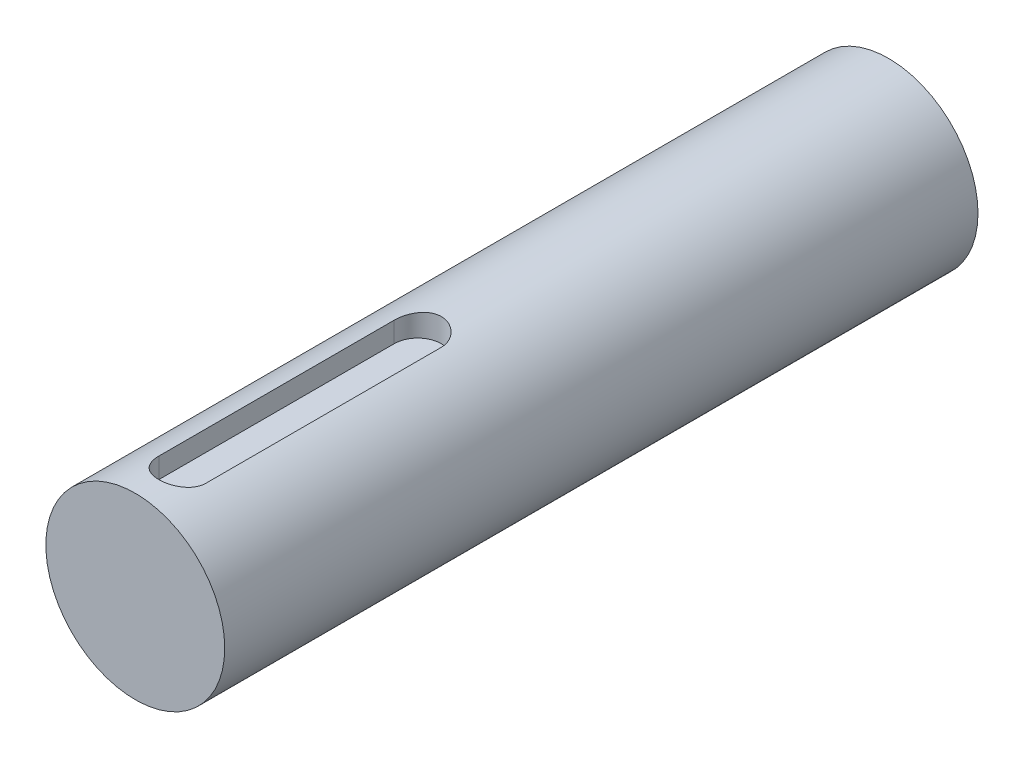
SolidWorks part; units mm, degrees
ref_plane "Front Plane" through (0, 0, 0) normal (0, 0, 1) x (1, 0, 0)
ref_plane "Top Plane" through (0, 0, 0) normal (0, 1, 0) x (1, 0, 0)
ref_plane "Right Plane" through (0, 0, 0) normal (1, 0, 0) x (0, 0, -1)
sketch "Sketch 1" plane through (0, 0, 0) normal (0, 0, 1) x (1, 0, 0)
  circle A0 centre (0, 0) radius 19
  dimension "D1" = 38
extrude "Boss-Extrude 1" add sketch "Sketch 1" along normal blind 160
ref_plane "Plane 1" through (0, 14, 0) normal (0, 1, 0) x (1, 0, 0)
sketch "Sketch 3" plane through (0, 14, 0) normal (0, 1, 0) x (1, 0, 0)
  line L0 (0, -33.0868) -> (0, -201.8775) construction
  line L1 (0, -150) -> (0, -100) construction
  line L2 (-5, -150) -> (-5, -100)
  line L3 (5, -150) -> (5, -100)
  line L4 (-19, -160) -> (19, -160) construction
  arc A0 (-5, -150) -> (5, -150) centre (0, -150) ccw
  arc A1 (5, -100) -> (-5, -100) centre (0, -100) ccw
  point P5 (0, -125)
  dimension "D1" = 10
  dimension "D2" = 60
  dimension "D3" = 50
extrude "Cut-Extrude 1" cut sketch "Sketch 3" along normal through all
